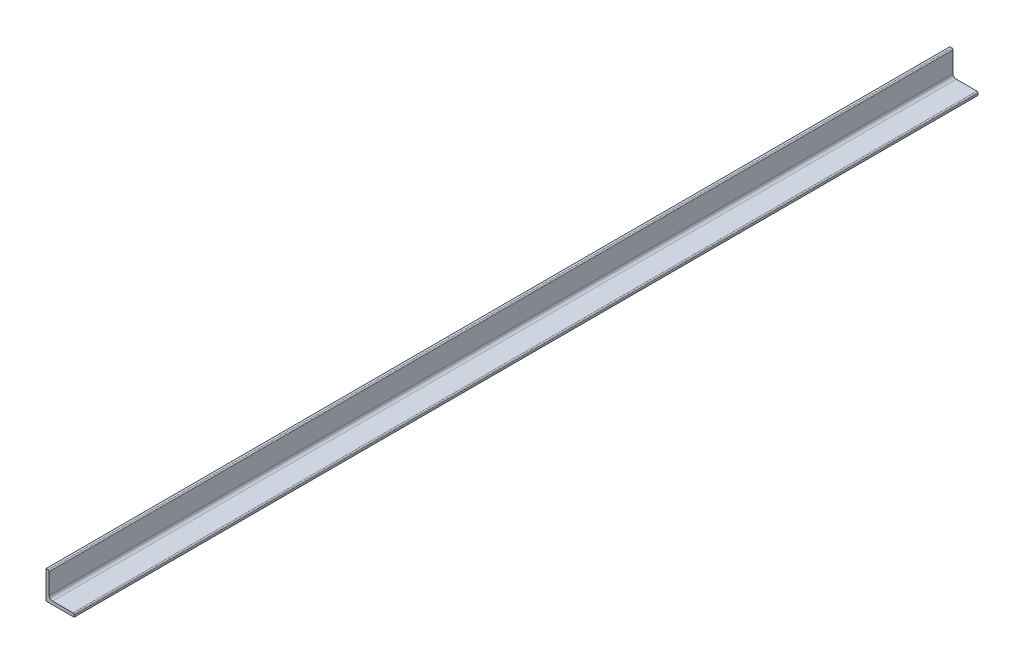
SolidWorks part; units mm, degrees
material "不锈钢角钢70×8/304"
ref_plane "Front Plane" through (0, 0, 0) normal (0, 0, 1) x (1, 0, 0)
ref_plane "Top Plane" through (0, 0, 0) normal (0, 1, 0) x (1, 0, 0)
ref_plane "Right Plane" through (0, 0, 0) normal (1, 0, 0) x (0, 0, -1)
sketch "Sketch1" plane through (0, 0, 0) normal (0, 0, 1) x (1, 0, 0)
  line L0 (0, 70) -> (0, 0)
  line L1 (0, 0) -> (70, 0)
  line L2 (70, 0) -> (70, 5)
  line L3 (67, 8) -> (16, 8)
  line L4 (8, 16) -> (8, 67)
  line L5 (5, 70) -> (0, 70)
  arc A0 (16, 8) -> (8, 16) centre (16, 16) cw
  arc A1 (70, 5) -> (67, 8) centre (67, 5) ccw
  arc A2 (8, 67) -> (5, 70) centre (5, 67) ccw
  dimension "D5" = 8
  dimension "D6" = 3
  dimension "D1" = 70
  dimension "D2" = 70
  dimension "D3" = 8
  dimension "D4" = 8
extrude "Boss-Extrude1" add sketch "Sketch1" along normal blind 2250
ref_plane "Plane1" through (0, 0, 0) normal (0.7071, 0.7071, 0) x (0, 0, -1)
